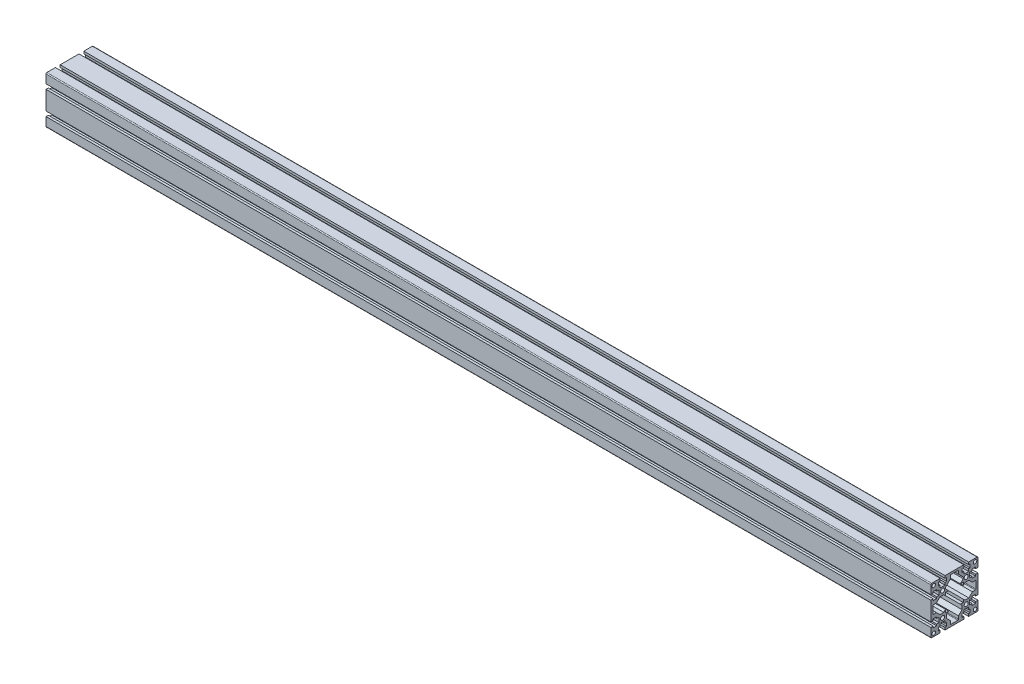
from build123d import *

# Parameters (mm, degrees)
SKETCH1_R                                = 3.4
SKETCH1_R_2                              = 3
ALUMINUM_PROFILE_80_X_80G_X_R1_5_1_DEPTH = 1500
SKETCH10_R                               = 3
CUT_EXTRUDE1_DEPTH                       = 1502.066287677


with BuildPart() as part:
    # Sketch1 → Aluminum profile 80 X 80G X R1.5(1) (new body)
    with BuildSketch(Plane.YZ.offset(-530.344827586)):
        with BuildLine():
            Line((-24.05, 40), (-24.05, 36))
            Line((-24.05, 36), (-26.75, 36))
            Line((-26.75, 36), (-26.75, 30))
            Line((-26.75, 30), (-24.05, 30))
            Line((-24.05, 30), (-24.05, 26))
            Line((-24.05, 26), (-15.95, 26))
            Line((-15.95, 26), (-15.95, 30))
            Line((-15.95, 30), (-13.25, 30))
            Line((-13.25, 30), (-13.25, 36))
            Line((-13.25, 36), (-15.95, 36))
            Line((-15.95, 36), (-15.95, 40))
            Line((-15.95, 40), (15.95, 40))
            Line((15.95, 40), (15.95, 36))
            Line((15.95, 36), (13.25, 36))
            Line((13.25, 36), (13.25, 30))
            Line((13.25, 30), (15.95, 30))
            Line((15.95, 30), (15.95, 26))
            Line((15.95, 26), (24.05, 26))
            Line((24.05, 26), (24.05, 30))
            Line((24.05, 30), (26.75, 30))
            Line((26.75, 30), (26.75, 36))
            Line((26.75, 36), (24.05, 36))
            Line((24.05, 36), (24.05, 40))
            Line((24.05, 40), (38.5, 40))
            ThreePointArc((38.5, 40), (39.560660172, 39.560660172), (40, 38.5))
            Line((40, 38.5), (40, 24.05))
            Line((40, 24.05), (36, 24.05))
            Line((36, 24.05), (36, 26.75))
            Line((36, 26.75), (30, 26.75))
            Line((30, 26.75), (30, 24.05))
            Line((30, 24.05), (26, 24.05))
            Line((26, 24.05), (26, 15.95))
            Line((26, 15.95), (30, 15.95))
            Line((30, 15.95), (30, 13.25))
            Line((30, 13.25), (36, 13.25))
            Line((36, 13.25), (36, 15.95))
            Line((36, 15.95), (40, 15.95))
            Line((40, 15.95), (40, -15.95))
            Line((40, -15.95), (36, -15.95))
            Line((36, -15.95), (36, -13.25))
            Line((36, -13.25), (30, -13.25))
            Line((30, -13.25), (30, -15.95))
            Line((30, -15.95), (26, -15.95))
            Line((26, -15.95), (26, -24.05))
            Line((26, -24.05), (30, -24.05))
            Line((30, -24.05), (30, -26.75))
            Line((30, -26.75), (36, -26.75))
            Line((36, -26.75), (36, -24.05))
            Line((36, -24.05), (40, -24.05))
            Line((40, -24.05), (40, -38.5))
            ThreePointArc((40, -38.5), (39.560660172, -39.560660172), (38.5, -40))
            Line((38.5, -40), (24.05, -40))
            Line((24.05, -40), (24.05, -36))
            Line((24.05, -36), (26.75, -36))
            Line((26.75, -36), (26.75, -30))
            Line((26.75, -30), (24.05, -30))
            Line((24.05, -30), (24.05, -26))
            Line((24.05, -26), (15.95, -26))
            Line((15.95, -26), (15.95, -30))
            Line((15.95, -30), (13.25, -30))
            Line((13.25, -30), (13.25, -36))
            Line((13.25, -36), (15.95, -36))
            Line((15.95, -36), (15.95, -40))
            Line((15.95, -40), (-15.95, -40))
            Line((-15.95, -40), (-15.95, -36))
            Line((-15.95, -36), (-13.25, -36))
            Line((-13.25, -36), (-13.25, -30))
            Line((-13.25, -30), (-15.95, -30))
            Line((-15.95, -30), (-15.95, -26))
            Line((-15.95, -26), (-24.05, -26))
            Line((-24.05, -26), (-24.05, -30))
            Line((-24.05, -30), (-26.75, -30))
            Line((-26.75, -30), (-26.75, -36))
            Line((-26.75, -36), (-24.05, -36))
            Line((-24.05, -36), (-24.05, -40))
            Line((-24.05, -40), (-38.5, -40))
            ThreePointArc((-38.5, -40), (-39.560660172, -39.560660172), (-40, -38.5))
            Line((-40, -38.5), (-40, -24.05))
            Line((-40, -24.05), (-36, -24.05))
            Line((-36, -24.05), (-36, -26.75))
            Line((-36, -26.75), (-30, -26.75))
            Line((-30, -26.75), (-30, -24.05))
            Line((-30, -24.05), (-26, -24.05))
            Line((-26, -24.05), (-26, -15.95))
            Line((-26, -15.95), (-30, -15.95))
            Line((-30, -15.95), (-30, -13.25))
            Line((-30, -13.25), (-36, -13.25))
            Line((-36, -13.25), (-36, -15.95))
            Line((-36, -15.95), (-40, -15.95))
            Line((-40, -15.95), (-40, 15.95))
            Line((-40, 15.95), (-36, 15.95))
            Line((-36, 15.95), (-36, 13.25))
            Line((-36, 13.25), (-30, 13.25))
            Line((-30, 13.25), (-30, 15.95))
            Line((-30, 15.95), (-26, 15.95))
            Line((-26, 15.95), (-26, 24.05))
            Line((-26, 24.05), (-30, 24.05))
            Line((-30, 24.05), (-30, 26.75))
            Line((-30, 26.75), (-36, 26.75))
            Line((-36, 26.75), (-36, 24.05))
            Line((-36, 24.05), (-40, 24.05))
            Line((-40, 24.05), (-40, 38.5))
            ThreePointArc((-40, 38.5), (-39.560660172, 39.560660172), (-38.5, 40))
            Line((-38.5, 40), (-24.05, 40))
        make_face()
        with Locations((-20, 20)):
            Circle(SKETCH1_R, mode=Mode.SUBTRACT)
        with Locations((20, 20)):
            Circle(SKETCH1_R, mode=Mode.SUBTRACT)
        with Locations((20, -20)):
            Circle(SKETCH1_R, mode=Mode.SUBTRACT)
        with Locations((-20, -20)):
            Circle(SKETCH1_R, mode=Mode.SUBTRACT)
        with Locations((-35, 35)):
            Circle(SKETCH1_R_2, mode=Mode.SUBTRACT)
        with Locations((35, 35)):
            Circle(SKETCH1_R_2, mode=Mode.SUBTRACT)
        with Locations((35, -35)):
            Circle(SKETCH1_R_2, mode=Mode.SUBTRACT)
        with BuildLine():
            Line((-13, 18), (-10, 15))
            Line((-10, 15), (-15, 15))
            Line((-15, 15), (-15, 10))
            Line((-15, 10), (-18, 13))
            Line((-18, 13), (-24.5, 13))
            Line((-24.5, 13), (-30.5, 7))
            Line((-30.5, 7), (-35.5, 7))
            ThreePointArc((-35.5, 7), (-36.207106781, 6.707106781), (-36.5, 6))
            Line((-36.5, 6), (-36.5, -6))
            ThreePointArc((-36.5, -6), (-36.207106781, -6.707106781), (-35.5, -7))
            Line((-35.5, -7), (-30.5, -7))
            Line((-30.5, -7), (-24.5, -13))
            Line((-24.5, -13), (-18, -13))
            Line((-18, -13), (-15, -10))
            Line((-15, -10), (-15, -15))
            Line((-15, -15), (-10, -15))
            Line((-10, -15), (-13, -18))
            Line((-13, -18), (-13, -24.5))
            Line((-13, -24.5), (-7, -30.5))
            Line((-7, -30.5), (-7, -35.5))
            ThreePointArc((-7, -35.5), (-6.707106781, -36.207106781), (-6, -36.5))
            Line((-6, -36.5), (6, -36.5))
            ThreePointArc((6, -36.5), (6.707106781, -36.207106781), (7, -35.5))
            Line((7, -35.5), (7, -30.5))
            Line((7, -30.5), (13, -24.5))
            Line((13, -24.5), (13, -18))
            Line((13, -18), (10, -15))
            Line((10, -15), (15, -15))
            Line((15, -15), (15, -10))
            Line((15, -10), (20, -15))
            Line((20, -15), (22.5, -15))
            Line((22.5, -15), (30.5, -7))
            Line((30.5, -7), (35.5, -7))
            ThreePointArc((35.5, -7), (36.207106781, -6.707106781), (36.5, -6))
            Line((36.5, -6), (36.5, 6))
            ThreePointArc((36.5, 6), (36.207106781, 6.707106781), (35.5, 7))
            Line((35.5, 7), (30.5, 7))
            Line((30.5, 7), (22.5, 15))
            Line((22.5, 15), (20, 15))
            Line((20, 15), (15, 10))
            Line((15, 10), (15, 15))
            Line((15, 15), (10, 15))
            Line((10, 15), (13, 18))
            Line((13, 18), (13, 24.5))
            Line((13, 24.5), (7, 30.5))
            Line((7, 30.5), (7, 35.5))
            ThreePointArc((7, 35.5), (6.707106781, 36.207106781), (6, 36.5))
            Line((6, 36.5), (-6, 36.5))
            ThreePointArc((-6, 36.5), (-6.707106781, 36.207106781), (-7, 35.5))
            Line((-7, 35.5), (-7, 30.5))
            Line((-7, 30.5), (-13, 24.5))
            Line((-13, 24.5), (-13, 18))
        make_face(mode=Mode.SUBTRACT)
    extrude(amount=ALUMINUM_PROFILE_80_X_80G_X_R1_5_1_DEPTH)

    # Sketch10 → Cut-Extrude1 (cut, through all)
    with BuildSketch(Plane(origin=(969.655172414, 0, 0), x_dir=(0, 0, -1), z_dir=(1, 0, 0))):
        with Locations((35, -35)):
            Circle(SKETCH10_R)
    extrude(amount=-CUT_EXTRUDE1_DEPTH, mode=Mode.SUBTRACT)


solid = part.part
